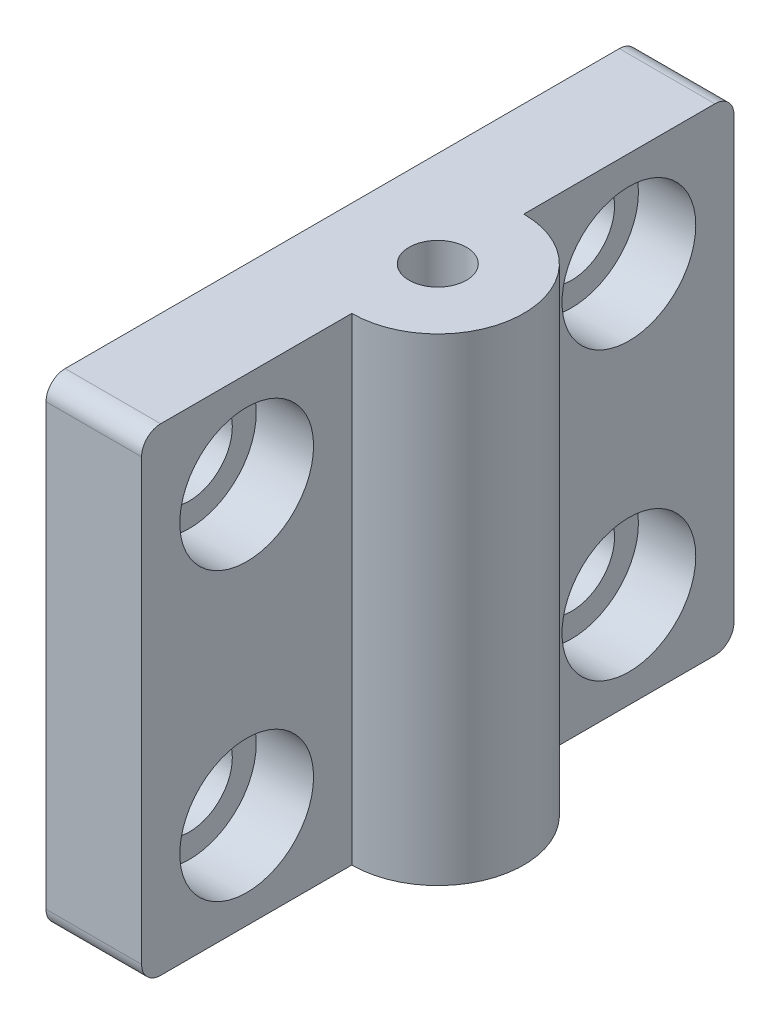
SolidWorks part; units mm, degrees
ref_plane "前视" through (0, 0, 0) normal (0, 0, 1) x (1, 0, 0)
ref_plane "上视" through (0, 0, 0) normal (0, 1, 0) x (1, 0, 0)
ref_plane "右视" through (0, 0, 0) normal (1, 0, 0) x (0, 0, -1)
sketch "草图1" plane through (0, 0, 0) normal (0, 1, 0) x (1, 0, 0)
  line L0 (10, -9) -> (10, -31)
  line L1 (0, 31) -> (10, 31)
  line L2 (0, 31) -> (0, -31)
  line L3 (0, -31) -> (10, -31)
  line L4 (10, 31) -> (10, 9)
  arc A0 (10, -9) -> (10, 9) centre (10, 0) ccw
  circle A1 centre (10, 0) radius 3
  dimension "D1" = 10
  dimension "D3" = 18
  dimension "D4" = 6
  dimension "D2" = 62
extrude "凸台-拉伸1" add sketch "草图1" along normal mid plane 50
hole_wizard "M8 六角凹头螺钉的柱形沉头孔1" positions "草图3" profile "草图2" counterbore size "M8" standard "Iso" end condition through all
sketch "草图3" plane through (10, 0, 0) normal (1, 0, 0) x (0, 0, -1)
  line L0 (0, 0) -> (0, 34.7151) construction
  line L2 (0, 0) -> (-43.2011, 0) construction
  point P0 (-20, 15)
  point P12 (-20, -15)
  point P13 (20, -15)
  point P14 (20, 15)
  dimension "D1" = 40
  dimension "D2" = 30
sketch "草图2" plane through (10, 15, 20) normal (0, 1, 0) x (0, 0, -1)
  line L0 (0, 0) -> (0, 10)
  line L1 (0, 10) -> (4.5, 10)
  line L3 (4.5, 10) -> (4.5, 6)
  line L4 (4.5, 6) -> (7, 6)
  line L5 (7, 6) -> (7, 0)
  line L7 (7, 0) -> (0, 0)
  line L11 (0, -6.35) -> (0, 107.95) construction
  dimension "通孔孔直径" = 9
  dimension "通孔孔深度" = 10
  dimension "柱形沉头孔直径" = 14
  dimension "柱形沉头孔深度" = 6
fillet "圆角1" radius 2 4 edges at (5, -25, 31) (5, -25, -31) (5, 25, -31) (5, 25, 31)
